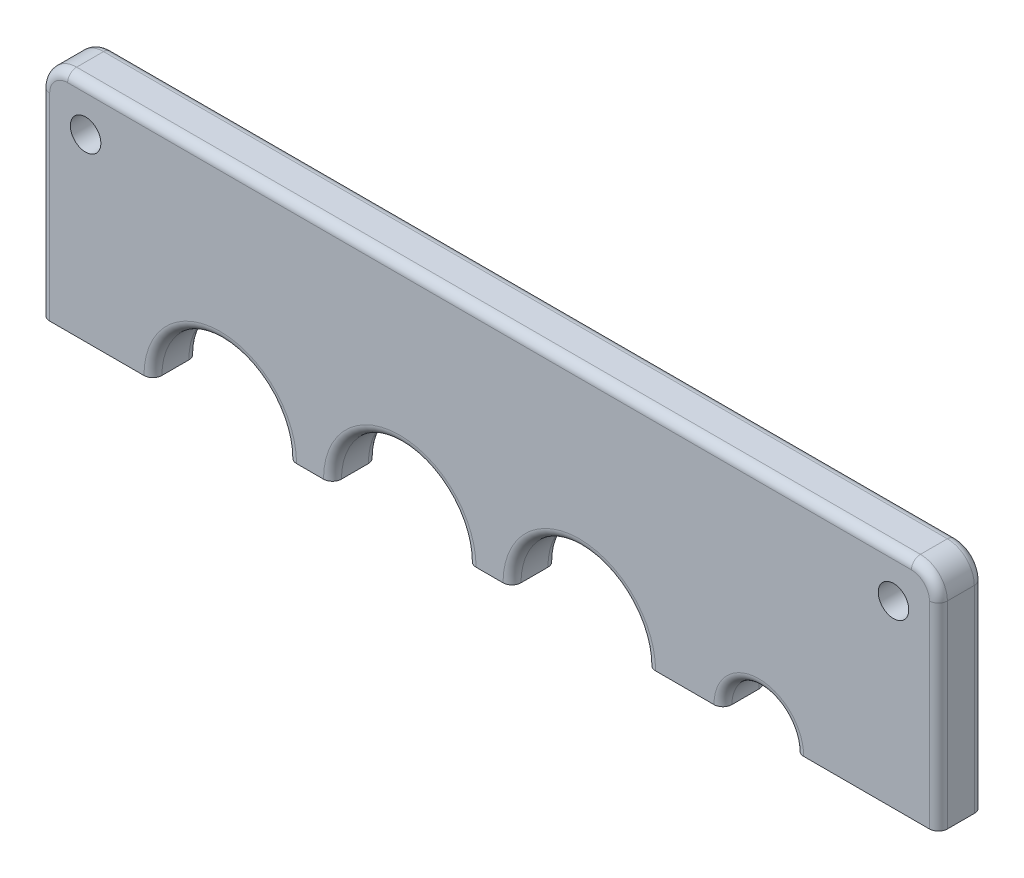
from build123d import *

# Parameters (mm, degrees)
SKETCH_1_W                   = 100
SKETCH_1_H                   = 25
EXTRUDE_1_DEPTH              = 5
SKETCH_2_R                   = 7.5
SKETCH_2_R_2                 = 4
CUT_EXTRUDE_1_DEPTH          = 104.198837203
HOLE_WIZARD_M3_1_D           = 3.4
HOLE_WIZARD_M3_1_CSINK_D     = 6.72
HOLE_WIZARD_M3_1_CSINK_ANGLE = 90
FILLET_1_R                   = 3
FILLET_2_R                   = 1


with BuildPart() as part:
    # 草图1 → 凸台-拉伸1 (new body)
    with BuildSketch(Plane.XY):
        with Locations((50, 12.5)):
            Rectangle(SKETCH_1_W, SKETCH_1_H)
    extrude(amount=EXTRUDE_1_DEPTH)

    # 草图2 → 切除-拉伸1 (cut, through all)
    with BuildSketch(Plane.XY.offset(5)):
        with Locations((20, 0)):
            Circle(SKETCH_2_R)
        with Locations((40, 0)):
            Circle(SKETCH_2_R)
        with Locations((60, 0)):
            Circle(SKETCH_2_R)
        with Locations((80, 0)):
            Circle(SKETCH_2_R_2)
    extrude(amount=-CUT_EXTRUDE_1_DEPTH, mode=Mode.SUBTRACT)

    # M3 六角凹锥坑螺钉的锥形沉头孔1 (through all)
    with Locations(Plane(origin=(0, 0, 0), x_dir=(-1, 0, 0), z_dir=(0, 0, -1))):
        with Locations((-5, 20), (-95, 20)):
            CounterSinkHole(HOLE_WIZARD_M3_1_D / 2, HOLE_WIZARD_M3_1_CSINK_D / 2, counter_sink_angle=HOLE_WIZARD_M3_1_CSINK_ANGLE)

    # 圆角1
    fillet_1_edges = [part.edges().sort_by_distance(p)[0] for p in [
        (0, 25, 2.5),
        (100, 25, 2.5),
    ]]
    fillet(fillet_1_edges, radius=FILLET_1_R)

    # 圆角2
    fillet_2_edges = [part.edges().sort_by_distance(p)[0] for p in [
        (100, 11, 5),
        (20, 7.5, 5),
        (20, 7.5, 0),
        (40, 7.5, 5),
        (40, 7.5, 0),
        (60, 7.5, 5),
        (60, 7.5, 0),
        (80, 4, 5),
        (80, 4, 0),
        (100, 11, 0),
        (50, 25, 0),
        (50, 25, 5),
        (0, 11, 0),
        (0.878679656, 24.121320344, 0),
        (99.121320344, 24.121320344, 0),
        (0, 11, 5),
        (0.878679656, 24.121320344, 5),
        (99.121320344, 24.121320344, 5),
    ]]
    fillet(fillet_2_edges, radius=FILLET_2_R)


solid = part.part
